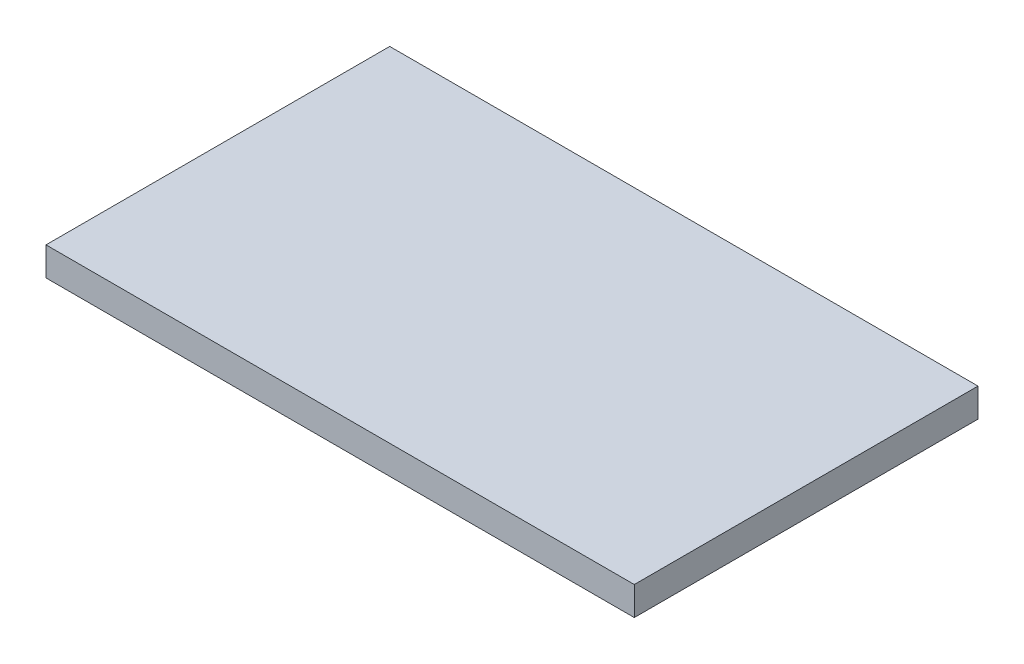
from build123d import *

# Parameters (mm, degrees)
BOSS_EXTRUDE1_DEPTH = 10


with BuildPart() as part:
    # Sketch1 → Boss-Extrude1 (new body)
    with BuildSketch(Plane(origin=(0, 0, 0), x_dir=(1, 0, 0), z_dir=(0, 1, 0))):
        Polygon((205.392105032, 120), (205.392105032, 0), (200, 0), (0, 0), (0, 120), (200, 120), align=None)
    extrude(amount=BOSS_EXTRUDE1_DEPTH)


solid = part.part
